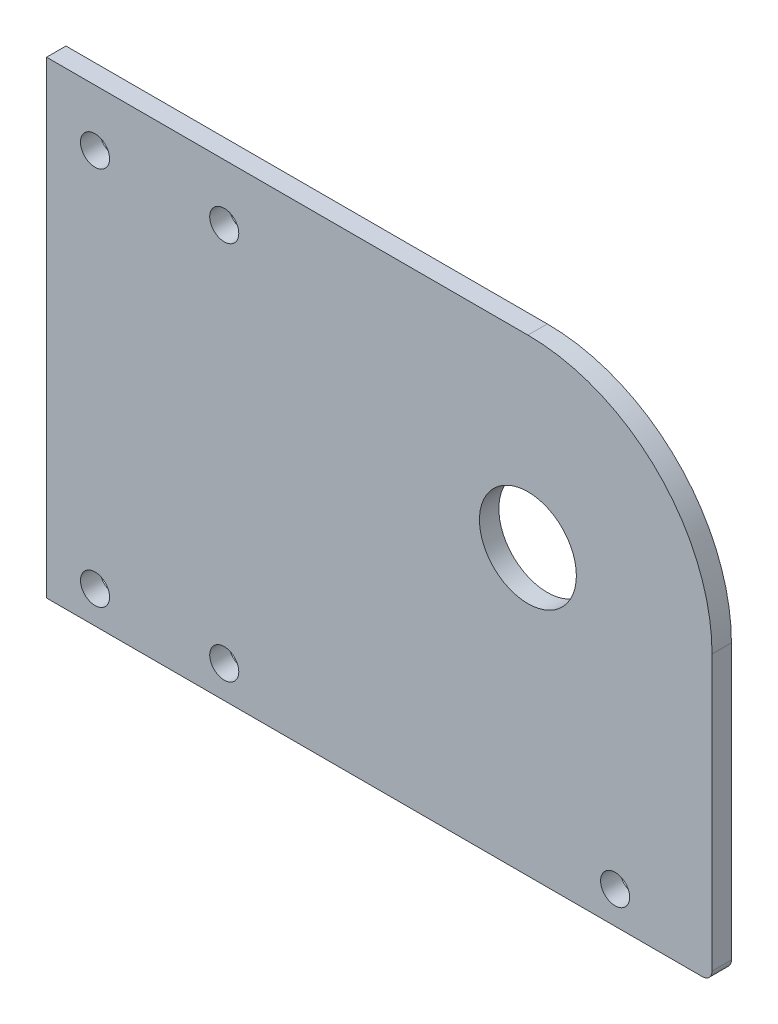
from build123d import *

# Parameters (mm, degrees)
SKETCH_1_W          = 206
SKETCH_1_H          = 145
EXTRUDE_1_DEPTH     = 6
SKETCH_3_R          = 4.5
CUT_EXTRUDE_2_DEPTH = 127.100158604
SKETCH_4_R          = 15
CUT_EXTRUDE_3_DEPTH = 127.100158604
FILLET_1_R          = 57
SKETCH_11_R         = 4.5
CUT_EXTRUDE_6_DEPTH = 127.100158604
FILLET_5_R          = 3


with BuildPart() as part:
    # 草图1 → 凸台-拉伸1 (new body)
    with BuildSketch(Plane.XY):
        Rectangle(SKETCH_1_W, SKETCH_1_H)
    extrude(amount=EXTRUDE_1_DEPTH)

    # 草图3 → 切除-拉伸2 (cut, through all)
    with BuildSketch(Plane.XY.offset(6)):
        with Locations((-88, 55)):
            Circle(SKETCH_3_R)
        with Locations((-48, 55)):
            Circle(SKETCH_3_R)
        with Locations((-88, -62.5)):
            Circle(SKETCH_3_R)
        with Locations((-48, -62.5)):
            Circle(SKETCH_3_R)
    extrude(amount=-CUT_EXTRUDE_2_DEPTH, mode=Mode.SUBTRACT)

    # 草图4 → 切除-拉伸3 (cut, through all)
    with BuildSketch(Plane.XY.offset(6)):
        with Locations((46, 15.5)):
            Circle(SKETCH_4_R)
    extrude(amount=-CUT_EXTRUDE_3_DEPTH, mode=Mode.SUBTRACT)

    # 圆角1
    fillet_1_edges = [part.edges().sort_by_distance(p)[0] for p in [
        (103, 72.5, 3),
    ]]
    fillet(fillet_1_edges, radius=FILLET_1_R)

    # 草图11 → 切除-拉伸6 (cut, through all)
    with BuildSketch(Plane.XY.offset(6)):
        with Locations((73, -62.5)):
            Circle(SKETCH_11_R)
    extrude(amount=-CUT_EXTRUDE_6_DEPTH, mode=Mode.SUBTRACT)

    # 圆角5
    fillet_5_edges = [part.edges().sort_by_distance(p)[0] for p in [
        (103, -72.5, 3),
    ]]
    fillet(fillet_5_edges, radius=FILLET_5_R)


solid = part.part
